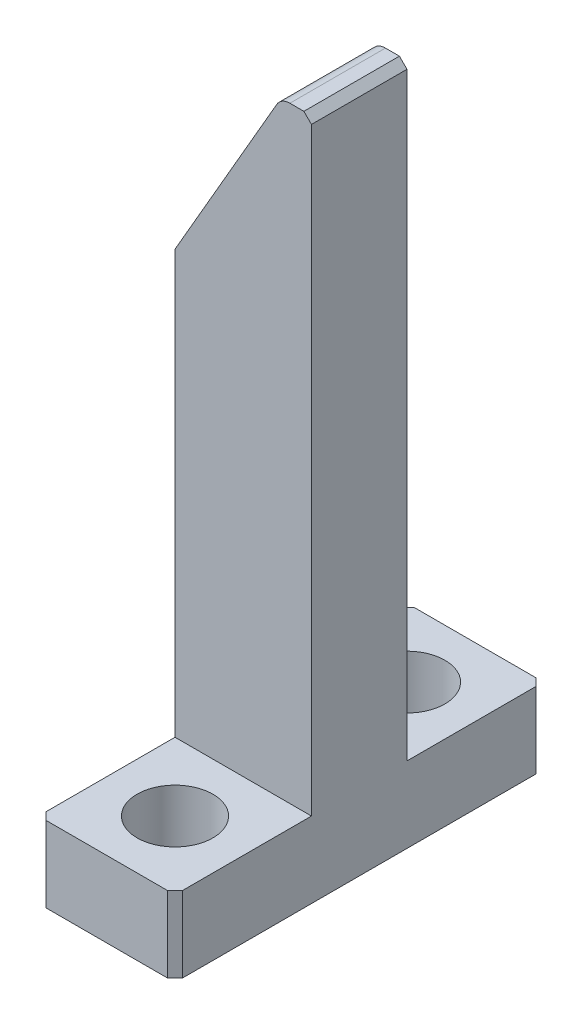
from build123d import *

# Parameters (mm, degrees)
SKETCH_1_W          = 9
SKETCH_1_H          = 40
EXTRUDE_1_DEPTH     = 6.3
SKETCH_2_W          = 9
SKETCH_2_H          = 24.3
EXTRUDE_2_DEPTH     = 5
CUT_EXTRUDE_1_DEPTH = 30.653667564
SKETCH_4_R          = 2.5
CUT_EXTRUDE_2_DEPTH = 44.062048256
FILLET_1_R          = 1
CHAMFER_2_SIZE      = 0.5


with BuildPart() as part:
    # 草图1 → 凸台-拉伸1 (new body)
    with BuildSketch(Plane.XY):
        Rectangle(SKETCH_1_W, SKETCH_1_H)
    extrude(amount=EXTRUDE_1_DEPTH)

    # 草图2 → 凸台-拉伸2 (add)
    with BuildSketch(Plane.XZ.offset(20)):
        with Locations((0, 3.15)):
            Rectangle(SKETCH_2_W, SKETCH_2_H)
    extrude(amount=EXTRUDE_2_DEPTH)

    # 草图3 → 切除-拉伸1 (cut, through all)
    with BuildSketch(Plane(origin=(0, 0, 0), x_dir=(-1, 0, 0), z_dir=(0, 0, -1))):
        Polygon((-2.5, 20), (4.5, 20), (4.5, 7.875644347), align=None)
    extrude(amount=-CUT_EXTRUDE_1_DEPTH, mode=Mode.SUBTRACT)

    # 草图4 → 切除-拉伸2 (cut, through all)
    with BuildSketch(Plane(origin=(0, -20, 0), x_dir=(1, 0, 0), z_dir=(0, 1, 0))):
        with Locations(Location((0, 4.5, 0), (0, 0, 270))):
            Circle(SKETCH_4_R)
        with Locations(Location((0, -10.8, 0), (0, 0, 270))):
            Circle(SKETCH_4_R)
    extrude(amount=-CUT_EXTRUDE_2_DEPTH, mode=Mode.SUBTRACT)

    # 圆角1
    fillet_1_edges = [part.edges().sort_by_distance(p)[0] for p in [
        (2.5, 20, 3.15),
    ]]
    fillet(fillet_1_edges, radius=FILLET_1_R)

    # 倒角2
    chamfer_2_edges = [part.edges().sort_by_distance(p)[0] for p in [
        (-4.5, -22.5, 15.3),
        (-4.5, -22.5, -9),
        (4.5, -22.5, -9),
        (4.5, -22.5, 15.3),
        (4.5, 20, 3.15),
    ]]
    chamfer(chamfer_2_edges, length=CHAMFER_2_SIZE)


solid = part.part
